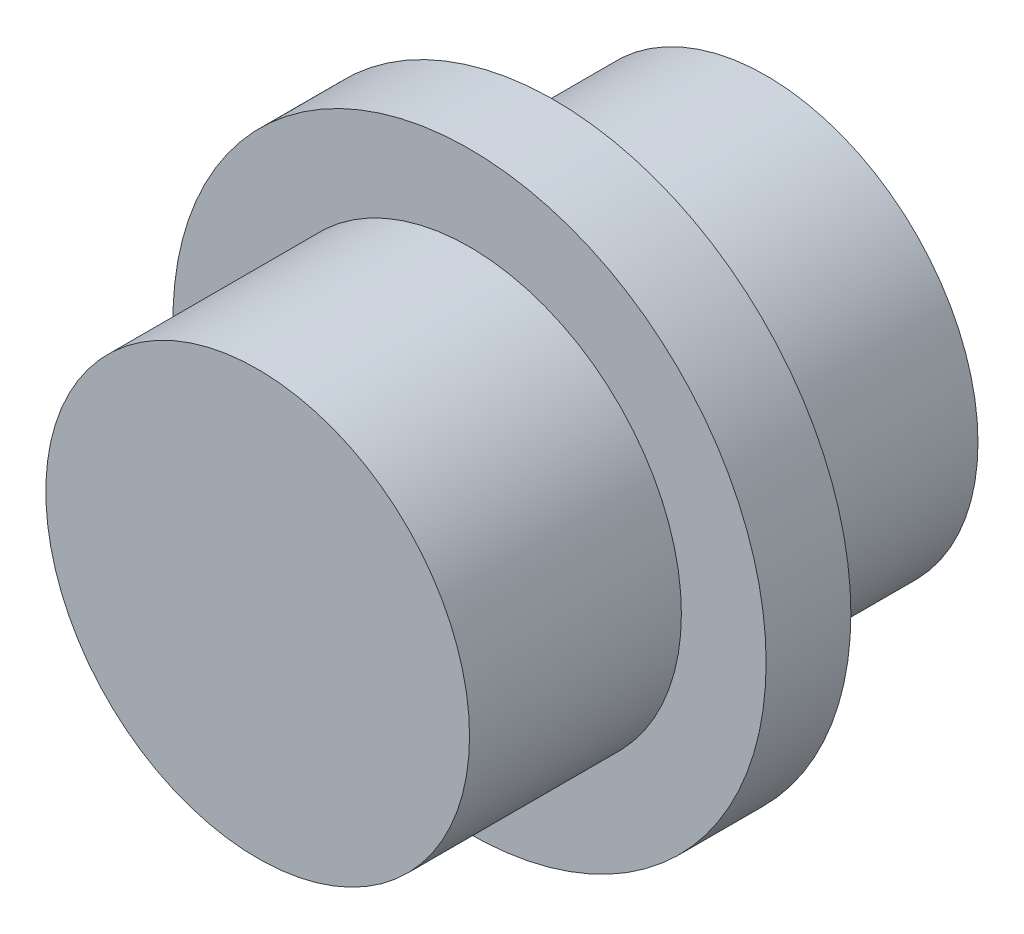
from build123d import *

# Parameters (mm, degrees)
SKETCH1_R           = 5
BOSS_EXTRUDE1_DEPTH = 5
SKETCH2_R           = 7
BOSS_EXTRUDE2_DEPTH = 2
SKETCH4_R           = 5
BOSS_EXTRUDE3_DEPTH = 5


with BuildPart() as part:
    # Sketch1 → Boss-Extrude1 (new body)
    with BuildSketch(Plane.XY):
        Circle(SKETCH1_R)
    extrude(amount=BOSS_EXTRUDE1_DEPTH)

    # Sketch2 → Boss-Extrude2 (add)
    with BuildSketch(Plane.XY.offset(5)):
        Circle(SKETCH2_R)
    extrude(amount=BOSS_EXTRUDE2_DEPTH)

    # Sketch4 → Boss-Extrude3 (add)
    with BuildSketch(Plane.XY.offset(7)):
        Circle(SKETCH4_R)
    extrude(amount=BOSS_EXTRUDE3_DEPTH)


solid = part.part
